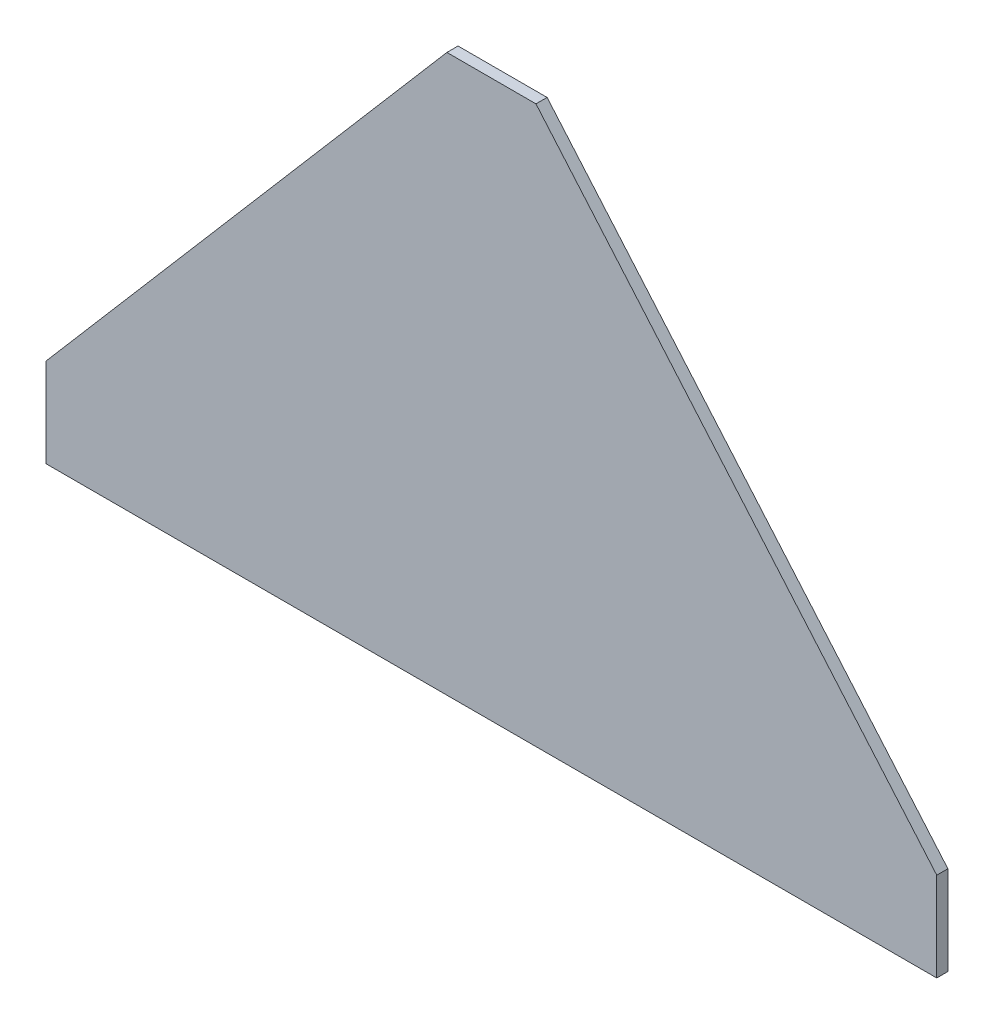
from build123d import *

# Parameters (mm, degrees)
SKETCH1_W           = 400
SKETCH1_H           = 250
BOSS_EXTRUDE1_DEPTH = 5
SKETCH2_OUTSIDE_W   = 496.346
SKETCH2_OUTSIDE_H   = 346.346
CUT_EXTRUDE1_DEPTH  = 5


with BuildPart() as part:
    # Sketch1 → Boss-Extrude1 (new body)
    with BuildSketch(Plane.XY):
        Rectangle(SKETCH1_W, SKETCH1_H)
    extrude(amount=BOSS_EXTRUDE1_DEPTH)

    # Sketch2 outside → Cut-Extrude1 (cut)
    with BuildSketch(Plane.XY.offset(5)):
        Rectangle(SKETCH2_OUTSIDE_W, SKETCH2_OUTSIDE_H)
        Polygon((-200, -85), (-20, 125), (20, 125), (200, -85), (200, -125), (-200, -125), align=None, mode=Mode.SUBTRACT)
    extrude(amount=-CUT_EXTRUDE1_DEPTH, mode=Mode.SUBTRACT)


solid = part.part
